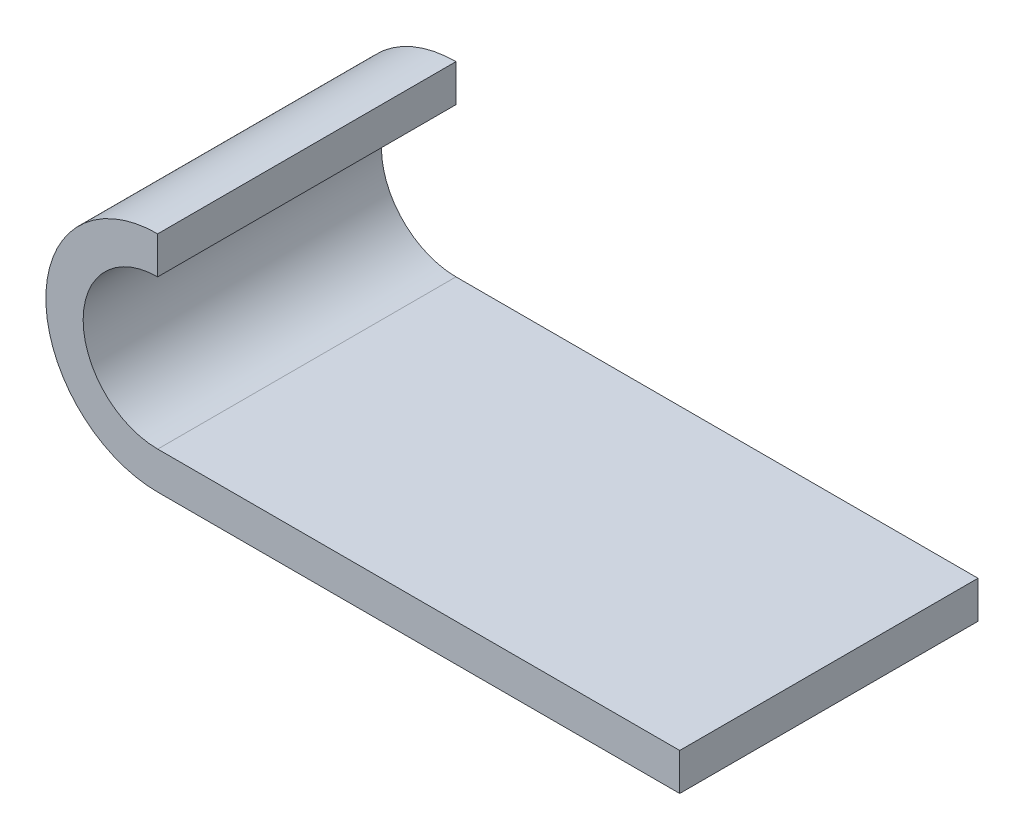
from build123d import *

# Parameters (mm, degrees)
BOSS_EXTRUDE1_DEPTH = 8


with BuildPart() as part:
    # Sketch1 → Boss-Extrude1 (new body)
    with BuildSketch(Plane.XY):
        with BuildLine():
            Line((-1.538253553, -40.507347935), (-15.538253553, -40.507347935))
            ThreePointArc((-15.538253553, -40.507347935), (-17.538253553, -38.507347935), (-15.538253553, -36.507347935))
            Line((-15.538253553, -36.507347935), (-15.538253553, -35.507347935))
            ThreePointArc((-15.538253553, -35.507347935), (-18.538253553, -38.507347935), (-15.538253553, -41.507347935))
            Line((-15.538253553, -41.507347935), (-1.538253553, -41.507347935))
            Line((-1.538253553, -41.507347935), (-1.538253553, -40.507347935))
        make_face()
    extrude(amount=BOSS_EXTRUDE1_DEPTH)


solid = part.part
